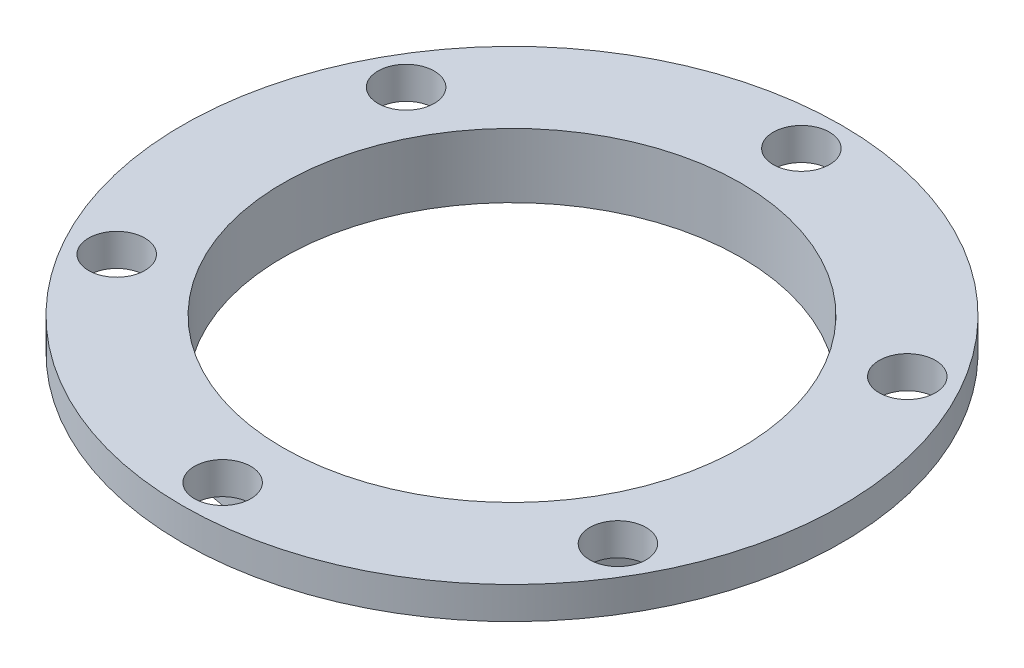
from build123d import *

# Parameters (mm, degrees)
SKETCH1_W                = 41
SKETCH1_H                = 4
SKETCH2_R                = 31
BOSS_EXTRUDE1_DEPTH      = 4
M52_CLEARANCE_HOLE1_D    = 57
F_7_0_7_DIAMETER_HOLE1_D = 7


with BuildPart() as part:
    # Sketch1 → Revolve1 (revolve)
    with BuildSketch(Plane.XY.offset(89.5), mode=Mode.PRIVATE) as revolve1_sk:
        with Locations((-1049.091991574, 72.472431577)):
            Rectangle(SKETCH1_W, SKETCH1_H)
    revolve(revolve1_sk.sketch.rotate(Axis((-1069.591991574, 74.472431577, 89.5), (0, -1, 0)), 270), axis=Axis((-1069.591991574, 74.472431577, 89.5), (0, -1, 0)))

    # Sketch2 → Boss-Extrude1 (add)
    with BuildSketch(Plane.XZ.offset(-70.472431577)):
        with Locations(Location((-1069.591991574, 89.5, 0), (0, 0, 270))):
            Circle(SKETCH2_R)
    extrude(amount=BOSS_EXTRUDE1_DEPTH)

    # M52 Clearance Hole1 (through all)
    with Locations(Plane(origin=(0, 66.472431577, 0), x_dir=(-1, 0, 0), z_dir=(0, -1, 0))):
        with Locations((1069.591991574, -89.5)):
            Hole(M52_CLEARANCE_HOLE1_D / 2)

    # Ø7.0 (7) Diameter Hole1 (through all)
    with Locations(Plane(origin=(0, 70.472431577, 0), x_dir=(-1, 0, 0), z_dir=(0, -1, 0))):
        with Locations((1069.591991574, -125.5), (1100.76890611, -107.5), (1100.76890611, -71.5), (1069.591991574, -53.5), (1038.415077038, -71.5), (1038.415077038, -107.5)):
            Hole(F_7_0_7_DIAMETER_HOLE1_D / 2)


solid = part.part
